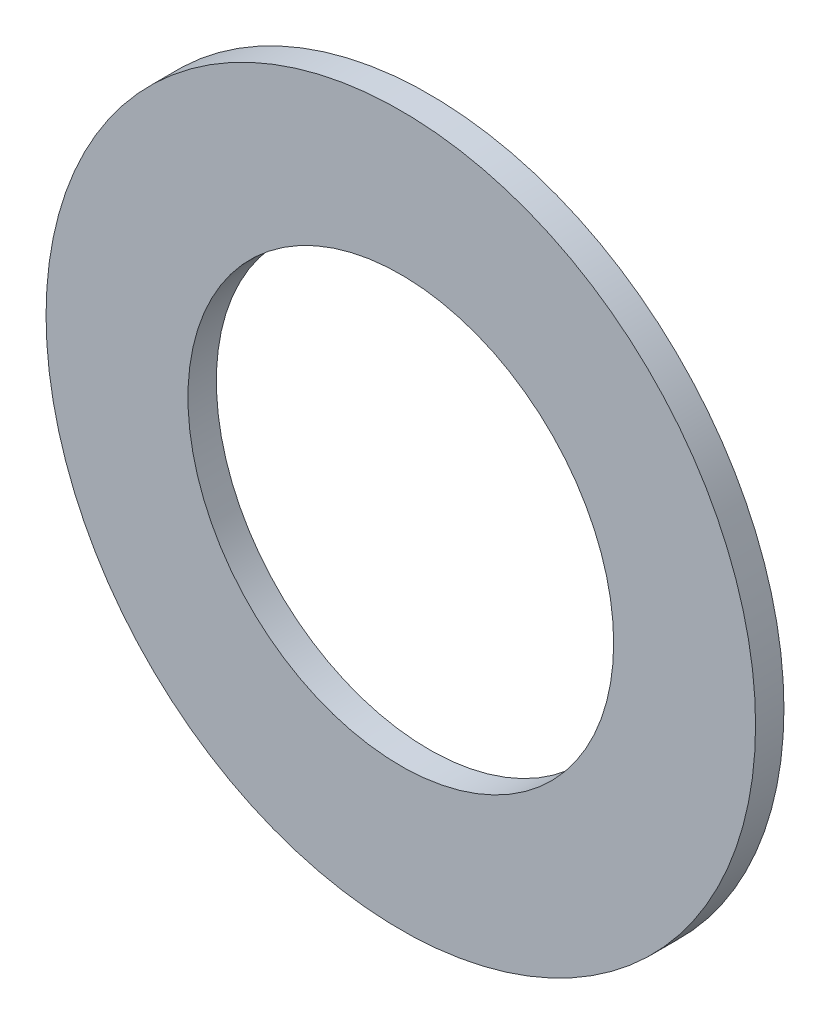
SolidWorks part; units mm, degrees
ref_plane "Front Plane" through (0, 0, 0) normal (0, 0, 1) x (1, 0, 0)
ref_plane "Top Plane" through (0, 0, 0) normal (0, 1, 0) x (1, 0, 0)
ref_plane "Right Plane" through (0, 0, 0) normal (1, 0, 0) x (0, 0, -1)
other "Configuration Table"
sketch "Sketch1" plane through (0, 0, 0) normal (0, 0, 1) x (1, 0, 0)
  circle A0 centre (0, 0) radius 1.5
  circle A1 centre (0, 0) radius 2.5
  dimension "D1" = 3
  dimension "D2" = 5
extrude "Boss-Extrude1" add sketch "Sketch1" along normal blind 0.2
